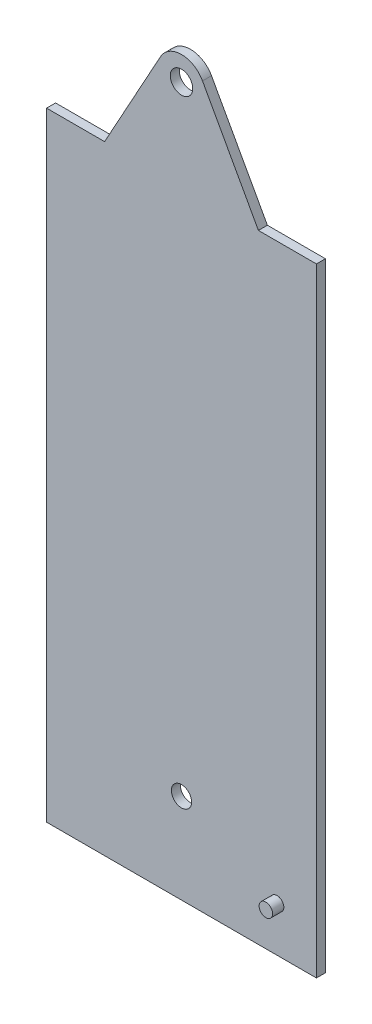
SolidWorks part; units mm, degrees
ref_plane "Front Plane" through (0, 0, 0) normal (0, 0, 1) x (1, 0, 0)
ref_plane "Top Plane" through (0, 0, 0) normal (0, 1, 0) x (1, 0, 0)
ref_plane "Right Plane" through (0, 0, 0) normal (1, 0, 0) x (0, 0, -1)
other "Configuration Table"
sketch "Sketch1" plane through (0, 0, 0) normal (0, 0, 1) x (1, 0, 0)
  line L0 (-120, 550) -> (-68.4, 550)
  line L1 (120, 550) -> (120, 0)
  line L2 (120, 0) -> (-120, 0)
  line L3 (-120, 0) -> (-120, 550)
  line L4 (-18.6842, 640.2882) -> (-68.4, 550)
  line L5 (18.6842, 640.2882) -> (68.4, 550)
  line L6 (68.4, 550) -> (120, 550)
  arc A0 (18.6842, 640.2882) -> (-18.6842, 640.2882) centre (0, 630) ccw
  circle A1 centre (0, 630) radius 10
  circle A2 centre (0, 80) radius 9
  point P2 (0, 0)
  dimension "D3" = 630
  dimension "D6" = 80
  dimension "D1" = 550
  dimension "D2" = 240
  dimension "D4" = 51.6
  dimension "D5" = 51.6
extrude "Boss-Extrude1" add sketch "Sketch1" along normal blind 8
sketch "Sketch2" plane through (0, 0, 8) normal (0, 0, 1) x (1, 0, 0)
  line L0 (120, 0) -> (120, 550) construction
  line L1 (-120, 0) -> (120, 0) construction
  circle A0 centre (85, 40) radius 6
  dimension "D1" = 35
  dimension "D2" = 40
extrude "Boss-Extrude2" add sketch "Sketch2" along normal blind 10
